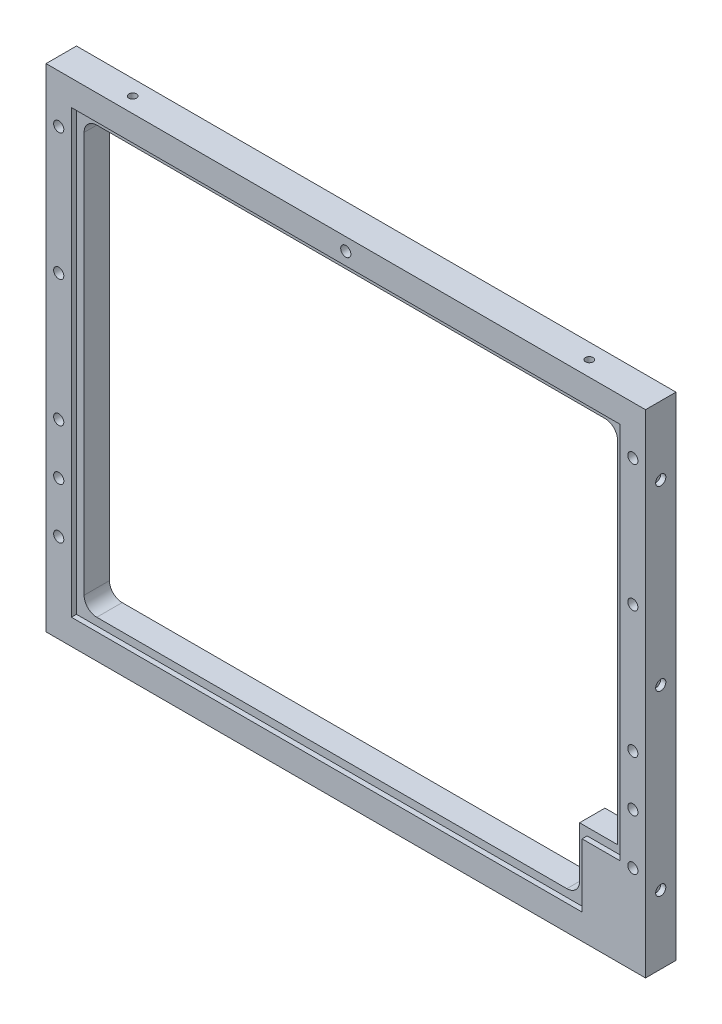
from build123d import *

# Parameters (mm, degrees)
SKETCH1_W           = 236.3
SKETCH1_H           = 194
BOSS_EXTRUDE1_DEPTH = 6
CUT_EXTRUDE1_DEPTH  = 2
CUT_EXTRUDE2_DEPTH  = 154.194068097
FILLET1_R           = 5
SKETCH4_R           = 2
CUT_EXTRUDE3_DEPTH  = 2
SKETCH5_R           = 1.5
CUT_EXTRUDE4_DEPTH  = 4
SKETCH7_R           = 2
CUT_EXTRUDE6_DEPTH  = 4
SKETCH8_R           = 2
CUT_EXTRUDE7_DEPTH  = 4


with BuildPart() as part:
    # Sketch1 → Boss-Extrude1 (new, symmetric)
    with BuildSketch(Plane.XY):
        Rectangle(SKETCH1_W, SKETCH1_H)
    extrude(amount=BOSS_EXTRUDE1_DEPTH, both=True)

    # Sketch2 → Cut-Extrude1 (cut)
    with BuildSketch(Plane.XY.offset(6)):
        Polygon((108.15, 87), (-108.15, 87), (-108.15, -87), (93.15, -87), (93.15, -62), (108.15, -62), align=None)
    extrude(amount=-CUT_EXTRUDE1_DEPTH, mode=Mode.SUBTRACT)

    # Sketch3 → Cut-Extrude2 (cut, through all)
    with BuildSketch(Plane.XY.offset(4)):
        Polygon((90.15, -84), (90.15, -59), (105.15, -59), (105.15, 84), (-105.15, 84), (-105.15, -84), align=None)
    extrude(amount=-CUT_EXTRUDE2_DEPTH, mode=Mode.SUBTRACT)

    # Fillet1
    fillet1_edges = [part.edges().sort_by_distance(p)[0] for p in [
        (90.15, -84, -1),
        (-105.15, -84, -1),
        (-105.15, 84, -1),
        (105.15, 84, -1),
    ]]
    fillet(fillet1_edges, radius=FILLET1_R)

    # Sketch4 → Cut-Extrude3 (cut)
    with BuildSketch(Plane.ZY.offset(118.15)):
        with Locations(Location((0, 0, 0), (0, 0, 270))):
            Circle(SKETCH4_R)
        with Locations(Location((0, 70, 0), (0, 0, 270))):
            Circle(SKETCH4_R)
        with Locations(Location((0, -70, 0), (0, 0, 90))):
            Circle(SKETCH4_R)
    cut_extrude3 = extrude(amount=-CUT_EXTRUDE3_DEPTH, mode=Mode.SUBTRACT)

    # Mirror1: Cut-Extrude3 across plane
    add(cut_extrude3.mirror(Plane(origin=(0, 0, 0), x_dir=(0, 0, 1), z_dir=(1, 0, 0))), mode=Mode.SUBTRACT)

    # Sketch5 → Cut-Extrude4 (cut)
    with BuildSketch(Plane(origin=(0, 97, 0), x_dir=(1, 0, 0), z_dir=(0, 1, 0))):
        with Locations(Location((-90, 0, 0), (0, 0, 270))):
            Circle(SKETCH5_R)
        with Locations(Location((90, 0, 0), (0, 0, 90))):
            Circle(SKETCH5_R)
    cut_extrude4 = extrude(amount=-CUT_EXTRUDE4_DEPTH, mode=Mode.SUBTRACT)

    # Mirror2: Cut-Extrude4 across plane
    add(cut_extrude4.mirror(Plane.ZX), mode=Mode.SUBTRACT)

    # Sketch7 → Cut-Extrude6 (cut)
    with BuildSketch(Plane.XY.offset(6)):
        with Locations((-113.15, 78)):
            Circle(SKETCH7_R)
        with Locations((-113.15, 28)):
            Circle(SKETCH7_R)
        with Locations((-113.15, -22)):
            Circle(SKETCH7_R)
        with Locations((-113.15, -42)):
            Circle(SKETCH7_R)
        with Locations((-113.15, -62)):
            Circle(SKETCH7_R)
    cut_extrude6 = extrude(amount=-CUT_EXTRUDE6_DEPTH, mode=Mode.SUBTRACT)

    # Mirror3: Cut-Extrude6 across plane
    add(cut_extrude6.mirror(Plane(origin=(0, 0, 0), x_dir=(0, 0, 1), z_dir=(1, 0, 0))), mode=Mode.SUBTRACT)

    # Sketch8 → Cut-Extrude7 (cut)
    with BuildSketch(Plane.XY.offset(6)):
        with Locations((0, 92)):
            Circle(SKETCH8_R)
    extrude(amount=-CUT_EXTRUDE7_DEPTH, mode=Mode.SUBTRACT)


solid = part.part
